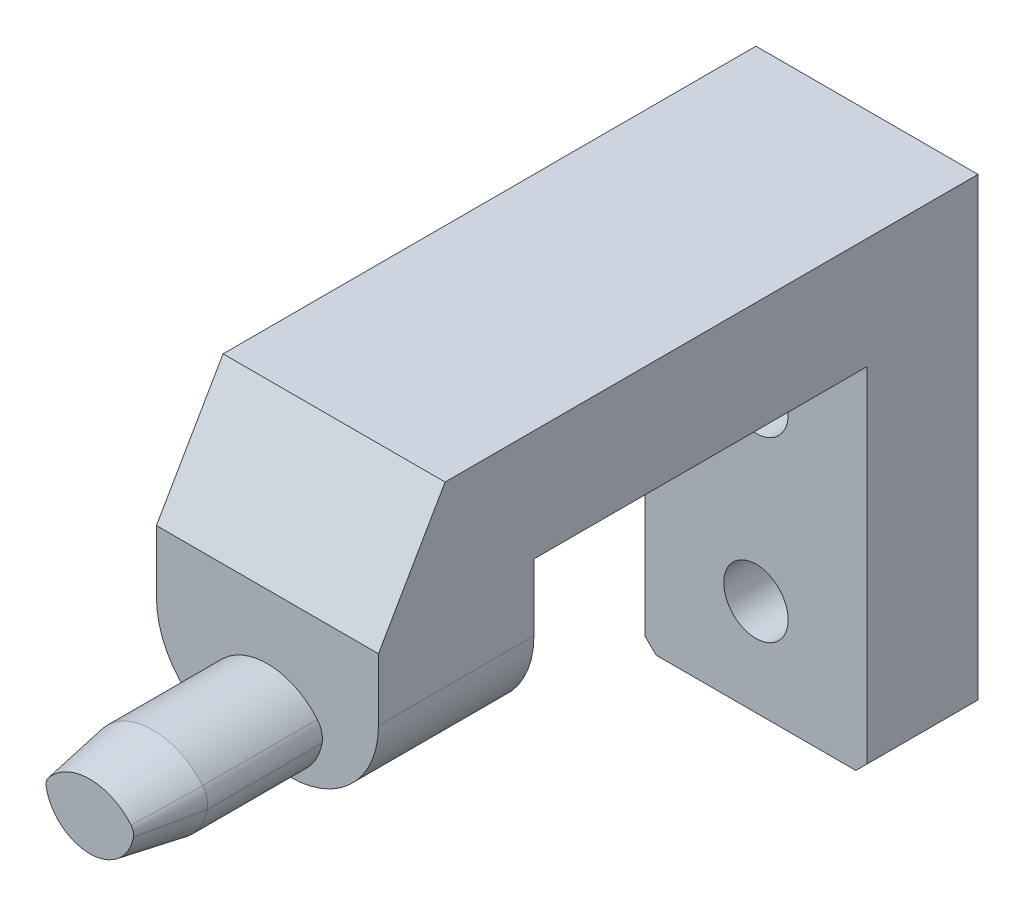
from build123d import *

# Parameters (mm, degrees)
SKETCH1_W              = 10
SKETCH1_H              = 20
BOSS_EXTRUDE1_DEPTH    = 5
SKETCH2_W              = 10
SKETCH2_H              = 5
BOSS_EXTRUDE2_DEPTH    = 16
M2_5_CLEARANCE_HOLE1_D = 2.9
SKETCH6_W              = 10
SKETCH6_H              = 12
BOSS_EXTRUDE4_DEPTH    = 7
CHAMFER1_SIZE          = 3
CHAMFER1_SIZE2         = 5.196152423
FILLET1_R              = 4
CHAMFER2_SIZE          = 0.5
BOSS_EXTRUDE6_DEPTH    = 8
FILLET3_R              = 1
CHAMFER3_SIZE          = 0.5
CHAMFER3_SIZE2         = 2.83564091
SKETCH9_R              = 2
CUT_EXTRUDE1_DEPTH     = 2.1


with BuildPart() as part:
    # Sketch1 → Boss-Extrude1 (new body)
    with BuildSketch(Plane(origin=(0, 0, 0), x_dir=(1, 0, 0), z_dir=(0, 1, 0))):
        Rectangle(SKETCH1_W, SKETCH1_H)
    extrude(amount=BOSS_EXTRUDE1_DEPTH)

    # Sketch2 → Boss-Extrude2 (add)
    with BuildSketch(Plane(origin=(0, 0, 0), x_dir=(-1, 0, 0), z_dir=(0, -1, 0))):
        with Locations((0, 7.5)):
            Rectangle(SKETCH2_W, SKETCH2_H)
    extrude(amount=BOSS_EXTRUDE2_DEPTH)

    # M2.5 Clearance Hole1 (through all)
    with Locations(Plane.XY.offset(-5)):
        with Locations((0, -11.65), (0, -3.65)):
            Hole(M2_5_CLEARANCE_HOLE1_D / 2)

    # Sketch6 → Boss-Extrude4 (add)
    with BuildSketch(Plane.XY.offset(10)):
        with Locations((0, -1)):
            Rectangle(SKETCH6_W, SKETCH6_H)
    extrude(amount=BOSS_EXTRUDE4_DEPTH)

    # Chamfer1
    chamfer1_edges = [part.edges().sort_by_distance(p)[0] for p in [
        (0, 5, 17),
    ]]
    chamfer1_side = [part.faces().sort_by_distance(p)[0] for p in [
        (0, 5, 3.5),
    ]]
    chamfer(chamfer1_edges, length=CHAMFER1_SIZE, length2=CHAMFER1_SIZE2, reference=chamfer1_side[0])

    # Fillet1
    fillet1_edges = [part.edges().sort_by_distance(p)[0] for p in [
        (5, -7, 13.5),
        (-5, -7, 13.5),
    ]]
    fillet(fillet1_edges, radius=FILLET1_R)

    # Chamfer2
    chamfer2_edges = [part.edges().sort_by_distance(p)[0] for p in [
        (5, -16, -7.5),
        (-5, -16, -7.5),
    ]]
    chamfer(chamfer2_edges, length=CHAMFER2_SIZE)

    # Sketch8 → Boss-Extrude6 (add)
    with BuildSketch(Plane.XY.offset(17)):
        with BuildLine():
            ThreePointArc((-2.5, -4.5), (0, -7), (2.5, -4.5))
            ThreePointArc((2.5, -4.5), (0, -3.084524053), (-2.5, -4.5))
        make_face()
    extrude(amount=BOSS_EXTRUDE6_DEPTH)

    # Fillet3
    fillet3_edges = [part.edges().sort_by_distance(p)[0] for p in [
        (2.5, -4.5, 21),
        (-2.5, -4.5, 21),
    ]]
    fillet(fillet3_edges, radius=FILLET3_R)

    # Chamfer3
    chamfer3_edges = [part.edges().sort_by_distance(p)[0] for p in [
        (0, -3.084524053, 25),
        (0, -7, 25),
        (-2.442268543, -4.526279661, 25),
        (2.442268543, -4.526279661, 25),
    ]]
    chamfer3_side = [part.faces().sort_by_distance(p)[0] for p in [
        (0, -5.00792315, 25),
    ]]
    chamfer(chamfer3_edges, length=CHAMFER3_SIZE, length2=CHAMFER3_SIZE2, reference=chamfer3_side[0])

    # Sketch9 → Cut-Extrude1 (cut)
    with BuildSketch(Plane(origin=(0, 0, -10), x_dir=(-1, 0, 0), z_dir=(0, 0, -1))):
        with Locations((0, -3.65)):
            Circle(SKETCH9_R)
        with Locations((0, -11.65)):
            Circle(SKETCH9_R)
    extrude(amount=-CUT_EXTRUDE1_DEPTH, mode=Mode.SUBTRACT)


solid = part.part
